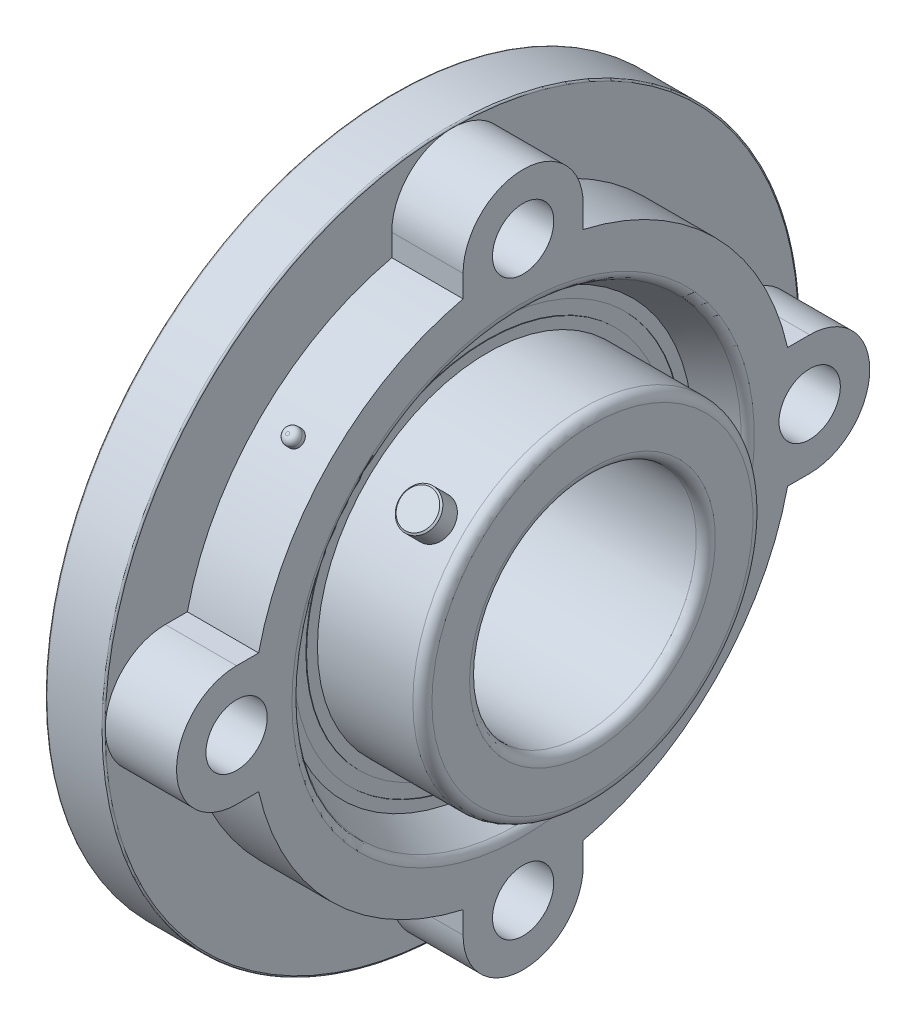
from build123d import *

# Parameters (mm, degrees)
SKETCH_2_2_R        = 9.459058326
SKETCH_2_2_R_2      = 71.368262753
BOSS_EXTRUDE1_DEPTH = 22
CUT_EXTRUDE1_START  = -18
SKETCH_2_2_2_R      = 9.459058326
CUT_EXTRUDE1_DEPTH  = 18
SKETCH3_W           = 2.5
SKETCH3_H           = 5.4
FILLET2_R           = 2


with BuildPart() as part:
    # Sketch1 → Revolve1 (revolve)
    with BuildSketch(Plane.XY, mode=Mode.PRIVATE) as revolve1_sk:
        with BuildLine():
            Line((-0.3, 63), (17.7, 63))
            ThreePointArc((17.7, 63), (18.053553391, 62.853553391), (18.2, 62.5))
            Line((18.2, 62.5), (18.2, 53))
            ThreePointArc((18.2, 53), (18.053553391, 52.646446609), (17.7, 52.5))
            Line((17.7, 52.5), (2.94, 52.5))
            ThreePointArc((2.94, 52.5), (0.861106063, 51.638893937), (0, 49.56))
            Line((0, 49.56), (0, 37.94))
            ThreePointArc((0, 37.94), (0.861106063, 35.861106063), (2.94, 35))
            Line((2.94, 35), (71.66, 35))
            ThreePointArc((71.66, 35), (73.738893937, 35.861106063), (74.6, 37.94))
            Line((74.6, 37.94), (74.6, 49.56))
            ThreePointArc((74.6, 49.56), (73.738893937, 51.638893937), (71.66, 52.5))
            Line((71.66, 52.5), (42.2, 52.5))
            Line((42.2, 52.5), (42.2, 55.864))
            Line((42.2, 55.864), (42, 55.864))
            Line((42, 55.864), (42, 59.956))
            Line((42, 59.956), (42.2, 59.956))
            Line((42.2, 59.956), (42.2, 63.32))
            Line((42.2, 63.32), (51.73, 68.822148065))
            ThreePointArc((51.73, 68.822148065), (52.806114687, 69.898262753), (53.2, 71.368262753))
            Line((53.2, 71.368262753), (53.2, 79))
            Line((53.2, 79), (31.2, 79))
            Line((31.2, 79), (31.2, 107))
            ThreePointArc((31.2, 107), (31.053553391, 107.353553391), (30.7, 107.5))
            Line((30.7, 107.5), (13.7, 107.5))
            ThreePointArc((13.7, 107.5), (13.346446609, 107.353553391), (13.2, 107))
            Line((13.2, 107), (13.2, 75.5))
            ThreePointArc((13.2, 75.5), (13.053553391, 75.146446609), (12.7, 75))
            Line((12.7, 75), (-0.3, 75))
            ThreePointArc((-0.3, 75), (-0.653553391, 74.853553391), (-0.8, 74.5))
            Line((-0.8, 74.5), (-0.8, 63.5))
            ThreePointArc((-0.8, 63.5), (-0.653553391, 63.146446609), (-0.3, 63))
        make_face()
    revolve(revolve1_sk.sketch.rotate(Axis((0, 0, 0), (1, 0, 0)), 90), axis=Axis((0, 0, 0), (1, 0, 0)))

    # Sketch 2_2 → Boss-Extrude1 (add)
    with BuildSketch(Plane(origin=(31.2, 0, 0), x_dir=(0, 0, -1), z_dir=(1, 0, 0))):
        with BuildLine():
            Line((-18.540941674, 88.459058326), (-18.540941674, 81.65088815))
            ThreePointArc((-18.540941674, 81.65088815), (-59.205717857, 59.205717857), (-81.65088815, 18.540941674))
            Line((-81.65088815, 18.540941674), (-88.459058326, 18.540941674))
            ThreePointArc((-88.459058326, 18.540941674), (-107, 0), (-88.459058326, -18.540941674))
            Line((-88.459058326, -18.540941674), (-81.65088815, -18.540941674))
            ThreePointArc((-81.65088815, -18.540941674), (-59.205717857, -59.205717857), (-18.540941674, -81.65088815))
            Line((-18.540941674, -81.65088815), (-18.540941674, -88.459058326))
            ThreePointArc((-18.540941674, -88.459058326), (0, -107), (18.540941674, -88.459058326))
            Line((18.540941674, -88.459058326), (18.540941674, -81.65088815))
            ThreePointArc((18.540941674, -81.65088815), (59.205717857, -59.205717857), (81.65088815, -18.540941674))
            Line((81.65088815, -18.540941674), (88.459058326, -18.540941674))
            ThreePointArc((88.459058326, -18.540941674), (107, 0), (88.459058326, 18.540941674))
            Line((88.459058326, 18.540941674), (81.65088815, 18.540941674))
            ThreePointArc((81.65088815, 18.540941674), (59.205717857, 59.205717857), (18.540941674, 81.65088815))
            Line((18.540941674, 81.65088815), (18.540941674, 88.459058326))
            ThreePointArc((18.540941674, 88.459058326), (0, 107), (-18.540941674, 88.459058326))
        make_face()
        with Locations((0, 88.459058326)):
            Circle(SKETCH_2_2_R, mode=Mode.SUBTRACT)
        with Locations(Location((88.459058326, 0, 0), (0, 0, 180))):
            Circle(SKETCH_2_2_R, mode=Mode.SUBTRACT)
        with Locations((0, -88.459058326)):
            Circle(SKETCH_2_2_R, mode=Mode.SUBTRACT)
        with Locations(Location((-88.459058326, 0, 0), (0, 0, 180))):
            Circle(SKETCH_2_2_R, mode=Mode.SUBTRACT)
        Circle(SKETCH_2_2_R_2, mode=Mode.SUBTRACT)
    extrude(amount=BOSS_EXTRUDE1_DEPTH)

    # Sketch 2_2 2 → Cut-Extrude1 (cut)
    with BuildSketch(Plane(origin=(31.2, 0, 0), x_dir=(0, 0, -1), z_dir=(1, 0, 0)).offset(CUT_EXTRUDE1_START)):
        with Locations((0, 88.459058326)):
            Circle(SKETCH_2_2_2_R)
        with Locations(Location((88.459058326, 0, 0), (0, 0, 180))):
            Circle(SKETCH_2_2_2_R)
        with Locations((0, -88.459058326)):
            Circle(SKETCH_2_2_2_R)
        with Locations(Location((-88.459058326, 0, 0), (0, 0, 180))):
            Circle(SKETCH_2_2_2_R)
    extrude(amount=CUT_EXTRUDE1_DEPTH, mode=Mode.SUBTRACT)

    # Sketch3 → Revolve2 (revolve)
    with BuildSketch(Plane(origin=(0, 0, 0), x_dir=(1, 0, 0), z_dir=(0, -0.7071067811865475, 0.7071067811865477)), mode=Mode.PRIVATE) as revolve2_sk:
        with Locations((43.35, 84.429529163)):
            Rectangle(SKETCH3_W, SKETCH3_H)
    revolve(revolve2_sk.sketch.rotate(Axis((42.1, 0, 0), (0, 0.7071067811865477, 0.7071067811865475)), 90), axis=Axis((42.1, 0, 0), (0, 0.7071067811865477, 0.7071067811865475)))

    # Sketch4 → Revolve3 (revolve)
    with BuildSketch(Plane(origin=(0, 0, 0), x_dir=(1, 0, 0), z_dir=(0, -0.7071067811865475, 0.7071067811865477)), mode=Mode.PRIVATE) as revolve3_sk:
        Polygon((62.6, 51.5), (62.6, 59.225), (68.1, 59.225), (68.6, 58.725), (68.6, 51.5), align=None)
    revolve(revolve3_sk.sketch.rotate(Axis((62.6, 0, 0), (0, 0.7071067811865476, 0.7071067811865475)), 90), axis=Axis((62.6, 0, 0), (0, 0.7071067811865476, 0.7071067811865475)))

    # Fillet2
    fillet2_edges = [part.edges().sort_by_distance(p)[0] for p in [
        (42.1, 59.84211396, 63.377647866),
    ]]
    fillet(fillet2_edges, radius=FILLET2_R)


solid = part.part
